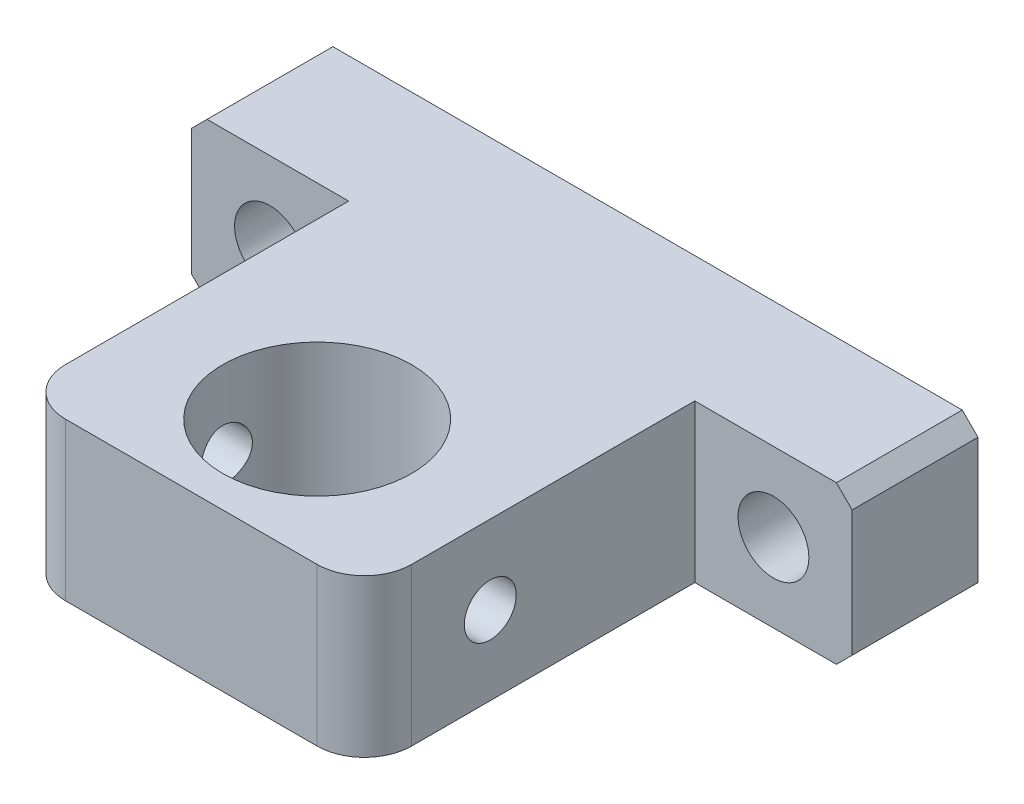
from build123d import *

# Parameters (mm, degrees)
SKETCH_1_W              = 42
SKETCH_1_H              = 10
EXTRUDE_1_DEPTH         = 8
SKETCH_2_W              = 22
SKETCH_2_H              = 10
EXTRUDE_2_DEPTH         = 21
SKETCH_3_R              = 6
CUT_EXTRUDE_1_DEPTH     = 38.175260591
HOLE_WIZARD_4_5_4_5_2_D = 4.5
HOLE_WIZARD_M4_1_D      = 3.3
FILLET_3_R              = 3
CHAMFER_1_SIZE          = 1


with BuildPart() as part:
    # 草图1 → 凸台-拉伸1 (new body)
    with BuildSketch(Plane.XY):
        Rectangle(SKETCH_1_W, SKETCH_1_H)
    extrude(amount=EXTRUDE_1_DEPTH)

    # 草图2 → 凸台-拉伸2 (add)
    with BuildSketch(Plane.XY.offset(8)):
        Rectangle(SKETCH_2_W, SKETCH_2_H)
    extrude(amount=EXTRUDE_2_DEPTH)

    # 草图3 → 切除-拉伸1 (cut, through all)
    with BuildSketch(Plane(origin=(0, 5, 0), x_dir=(1, 0, 0), z_dir=(0, 1, 0))):
        with Locations(Location((0, -21, 0), (0, 0, 270))):
            Circle(SKETCH_3_R)
    extrude(amount=-CUT_EXTRUDE_1_DEPTH, mode=Mode.SUBTRACT)

    # Ø4.5 (4.5) 直径孔2 (through all)
    with Locations(Plane.XY.offset(8)):
        with Locations((-16, 0), (16, 0)):
            Hole(HOLE_WIZARD_4_5_4_5_2_D / 2)

    # M4 螺纹孔1 (through all)
    with Locations(Plane(origin=(11, 0, 0), x_dir=(0, 0, -1), z_dir=(1, 0, 0))):
        with Locations((-21, 0)):
            Hole(HOLE_WIZARD_M4_1_D / 2)

    # 圆角3
    fillet_3_edges = [part.edges().sort_by_distance(p)[0] for p in [
        (-11, 0, 29),
        (11, 0, 29),
    ]]
    fillet(fillet_3_edges, radius=FILLET_3_R)

    # 倒角1
    chamfer_1_edges = [part.edges().sort_by_distance(p)[0] for p in [
        (21, -5, 4),
        (21, 5, 4),
        (-21, -5, 4),
        (-21, 5, 4),
    ]]
    chamfer(chamfer_1_edges, length=CHAMFER_1_SIZE)


solid = part.part
